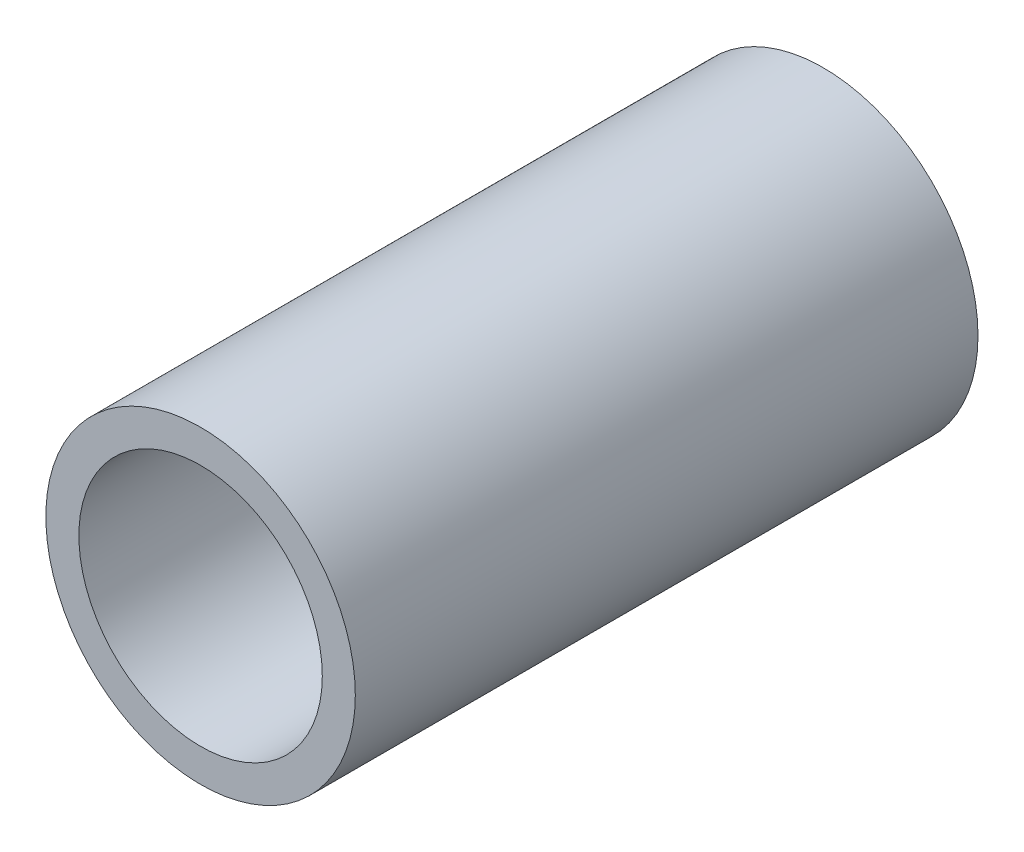
SolidWorks part; units mm, degrees
material "1023 Carbon steel plate (SS)"
ref_plane "Front Plane" through (0, 0, 0) normal (0, 0, 1) x (1, 0, 0)
ref_plane "Top Plane" through (0, 0, 0) normal (0, 1, 0) x (1, 0, 0)
ref_plane "Right Plane" through (0, 0, 0) normal (1, 0, 0) x (0, 0, -1)
sketch "Sketch1" plane through (0, 0, 0) normal (0, 0, 1) x (1, 0, 0)
  circle A0 centre (0, 0) radius 41.25
  circle A1 centre (0, 0) radius 32.45
  dimension "D1" = 82.5
  dimension "D2" = 64.9
extrude "Boss-Extrude1" add sketch "Sketch1" along normal blind 166
